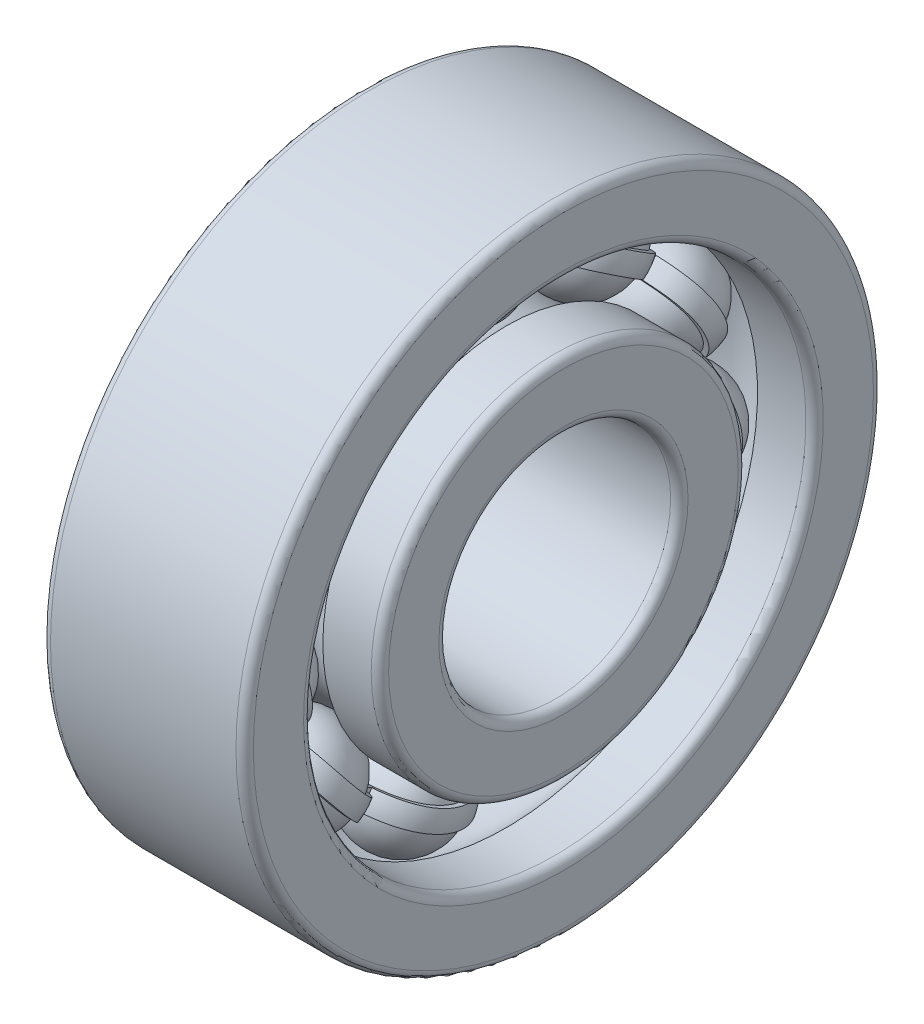
from build123d import *
from build123d.topology import SkipClean

# Parameters (mm, degrees)
SKETCH_5_W               = 1.05
SKETCH_5_H               = 0.7
PATTERN_CIRCULAR_5_COUNT = 11
PATTERN_CIRCULAR_2_COUNT = 11


with BuildPart() as part:
    # 草图2 → 旋转1 (revolve)
    with BuildSketch(Plane.XY, mode=Mode.PRIVATE) as revolve_1_sk:
        with BuildLine():
            Line((3.2, 4), (-3.2, 4))
            ThreePointArc((-3.2, 4), (-3.412132034, 4.087867966), (-3.5, 4.3))
            Line((-3.5, 4.3), (-3.5, 6.033333333))
            ThreePointArc((-3.5, 6.033333333), (-3.412132034, 6.245465368), (-3.2, 6.333333333))
            Line((-3.2, 6.333333333), (-1.304372987, 6.333333333))
            ThreePointArc((-1.304372987, 6.333333333), (0, 5.75), (1.304372987, 6.333333333))
            Line((1.304372987, 6.333333333), (3.2, 6.333333333))
            ThreePointArc((3.2, 6.333333333), (3.412132034, 6.245465368), (3.5, 6.033333333))
            Line((3.5, 6.033333333), (3.5, 4.3))
            ThreePointArc((3.5, 4.3), (3.412132034, 4.087867966), (3.2, 4))
        make_face()
        with BuildLine():
            Line((-3.5, 10.7), (-3.5, 8.966666667))
            ThreePointArc((-3.5, 8.966666667), (-3.412132034, 8.754534632), (-3.2, 8.666666667))
            Line((-3.2, 8.666666667), (-1.304372987, 8.666666667))
            ThreePointArc((-1.304372987, 8.666666667), (0, 9.25), (1.304372987, 8.666666667))
            Line((1.304372987, 8.666666667), (3.2, 8.666666667))
            ThreePointArc((3.2, 8.666666667), (3.412132034, 8.754534632), (3.5, 8.966666667))
            Line((3.5, 8.966666667), (3.5, 10.7))
            ThreePointArc((3.5, 10.7), (3.412132034, 10.912132034), (3.2, 11))
            Line((3.2, 11), (-3.2, 11))
            ThreePointArc((-3.2, 11), (-3.412132034, 10.912132034), (-3.5, 10.7))
        make_face()
    revolve(revolve_1_sk.sketch.rotate(Axis((-3.5, 0, 0), (1, 0, 0)), 90), axis=Axis((-3.5, 0, 0), (1, 0, 0)))


with BuildPart() as body_2:
    # 草图5 → 旋转3 (revolve)
    with BuildSketch(Plane.XY, mode=Mode.PRIVATE) as revolve_3_sk:
        with Locations((0, 7.5)):
            Rectangle(SKETCH_5_W, SKETCH_5_H)
    revolve(revolve_3_sk.sketch.rotate(Axis((-19.927092192, 0, 0), (1, 0, 0)), 90), axis=Axis((-19.927092192, 0, 0), (1, 0, 0)))



with BuildPart() as body_3:
    # 草图3 → 旋转2 (revolve)
    with BuildSketch(Plane.XY):
        with BuildLine():
            Line((-1.925, 7.5), (1.925, 7.5))
            ThreePointArc((1.925, 7.5), (0, 9.425), (-1.925, 7.5))
        make_face()
    revolve(axis=Axis((-1.925, 7.5, 0), (1, 0, 0)))


with BuildPart() as pattern_circular_5_1:
    # 阵列(圆周)5: pattern copy
    add(body_3.part.rotate(Axis((0, 0, 0), (1, 0, 0)), 1 * 360 / PATTERN_CIRCULAR_5_COUNT))


with BuildPart() as pattern_circular_5_2:
    # 阵列(圆周)5: pattern copy
    add(body_3.part.rotate(Axis((0, 0, 0), (1, 0, 0)), 2 * 360 / PATTERN_CIRCULAR_5_COUNT))


with BuildPart() as pattern_circular_5_3:
    # 阵列(圆周)5: pattern copy
    add(body_3.part.rotate(Axis((0, 0, 0), (1, 0, 0)), 3 * 360 / PATTERN_CIRCULAR_5_COUNT))


with BuildPart() as pattern_circular_5_4:
    # 阵列(圆周)5: pattern copy
    add(body_3.part.rotate(Axis((0, 0, 0), (1, 0, 0)), 4 * 360 / PATTERN_CIRCULAR_5_COUNT))


with BuildPart() as pattern_circular_5_5:
    # 阵列(圆周)5: pattern copy
    add(body_3.part.rotate(Axis((0, 0, 0), (1, 0, 0)), 5 * 360 / PATTERN_CIRCULAR_5_COUNT))


with BuildPart() as pattern_circular_5_6:
    # 阵列(圆周)5: pattern copy
    add(body_3.part.rotate(Axis((0, 0, 0), (1, 0, 0)), 6 * 360 / PATTERN_CIRCULAR_5_COUNT))


with BuildPart() as pattern_circular_5_7:
    # 阵列(圆周)5: pattern copy
    add(body_3.part.rotate(Axis((0, 0, 0), (1, 0, 0)), 7 * 360 / PATTERN_CIRCULAR_5_COUNT))


with BuildPart() as pattern_circular_5_8:
    # 阵列(圆周)5: pattern copy
    add(body_3.part.rotate(Axis((0, 0, 0), (1, 0, 0)), 8 * 360 / PATTERN_CIRCULAR_5_COUNT))


with BuildPart() as pattern_circular_5_9:
    # 阵列(圆周)5: pattern copy
    add(body_3.part.rotate(Axis((0, 0, 0), (1, 0, 0)), 9 * 360 / PATTERN_CIRCULAR_5_COUNT))


with BuildPart() as pattern_circular_5_10:
    # 阵列(圆周)5: pattern copy
    add(body_3.part.rotate(Axis((0, 0, 0), (1, 0, 0)), 10 * 360 / PATTERN_CIRCULAR_5_COUNT))


with BuildPart() as cut_revolve_1_tool:
    # 草图6 → 切除-旋转1 (revolve)
    with BuildSketch(Plane.XY):
        with BuildLine():
            Line((-1.89291442, 7.85), (1.89291442, 7.85))
            ThreePointArc((1.89291442, 7.85), (0, 9.425), (-1.89291442, 7.85))
        make_face()
        with BuildLine():
            Line((-1.89291442, 7.15), (1.89291442, 7.15))
            ThreePointArc((1.89291442, 7.15), (0, 5.575), (-1.89291442, 7.15))
        make_face()
    revolve(axis=Axis((-19.927092192, 0, 0), (1, 0, 0)))


with BuildPart() as part_1:
    add(part.part)

    # 切除-旋转1: cut by cut_revolve_1_tool
    add(cut_revolve_1_tool.part, mode=Mode.SUBTRACT)


with BuildPart() as body_3_1:
    add(body_3.part)

    # 切除-旋转1: cut by cut_revolve_1_tool
    add(cut_revolve_1_tool.part, mode=Mode.SUBTRACT)


with BuildPart() as pattern_circular_5_1_1:
    add(pattern_circular_5_1.part)

    # 切除-旋转1: cut by cut_revolve_1_tool
    add(cut_revolve_1_tool.part, mode=Mode.SUBTRACT)


with BuildPart() as pattern_circular_5_2_1:
    add(pattern_circular_5_2.part)

    # 切除-旋转1: cut by cut_revolve_1_tool
    add(cut_revolve_1_tool.part, mode=Mode.SUBTRACT)


with BuildPart() as pattern_circular_5_3_1:
    add(pattern_circular_5_3.part)

    # 切除-旋转1: cut by cut_revolve_1_tool
    add(cut_revolve_1_tool.part, mode=Mode.SUBTRACT)


with BuildPart() as pattern_circular_5_4_1:
    add(pattern_circular_5_4.part)

    # 切除-旋转1: cut by cut_revolve_1_tool
    add(cut_revolve_1_tool.part, mode=Mode.SUBTRACT)


with BuildPart() as pattern_circular_5_5_1:
    add(pattern_circular_5_5.part)

    # 切除-旋转1: cut by cut_revolve_1_tool
    add(cut_revolve_1_tool.part, mode=Mode.SUBTRACT)


with BuildPart() as pattern_circular_5_6_1:
    add(pattern_circular_5_6.part)

    # 切除-旋转1: cut by cut_revolve_1_tool
    add(cut_revolve_1_tool.part, mode=Mode.SUBTRACT)


with BuildPart() as pattern_circular_5_7_1:
    add(pattern_circular_5_7.part)

    # 切除-旋转1: cut by cut_revolve_1_tool
    add(cut_revolve_1_tool.part, mode=Mode.SUBTRACT)


with BuildPart() as pattern_circular_5_8_1:
    add(pattern_circular_5_8.part)

    # 切除-旋转1: cut by cut_revolve_1_tool
    add(cut_revolve_1_tool.part, mode=Mode.SUBTRACT)


with BuildPart() as pattern_circular_5_9_1:
    add(pattern_circular_5_9.part)

    # 切除-旋转1: cut by cut_revolve_1_tool
    add(cut_revolve_1_tool.part, mode=Mode.SUBTRACT)


with BuildPart() as pattern_circular_5_10_1:
    add(pattern_circular_5_10.part)

    # 切除-旋转1: cut by cut_revolve_1_tool
    add(cut_revolve_1_tool.part, mode=Mode.SUBTRACT)


with BuildPart() as body_2_1:
    with SkipClean():  # the faces are left unmerged after this step: merging them gives an invalid solid
        add(body_2.part)

        add(body_3_1.part)  # 旋转4 merges body 3
        # 草图7 → 旋转4 (revolve)
        with BuildSketch(Plane.XY):
            with BuildLine():
                Line((-1.75, 7.5), (1.75, 7.5))
                ThreePointArc((1.75, 7.5), (0, 9.25), (-1.75, 7.5))
            make_face()
        revolve_4 = revolve(axis=Axis((-1.75, 7.5, 0), (1, 0, 0)))

    # 阵列(圆周)2: 旋转4 ×11 about axis
    pattern_circular_2_axis = Axis((0, 0, 0), (1, 0, 0))
    for i in range(1, PATTERN_CIRCULAR_2_COUNT):
        add(revolve_4.rotate(pattern_circular_2_axis, i * 360 / PATTERN_CIRCULAR_2_COUNT))


solid = Compound([part_1.part, pattern_circular_5_1_1.part, pattern_circular_5_2_1.part, pattern_circular_5_3_1.part, pattern_circular_5_4_1.part, pattern_circular_5_5_1.part, pattern_circular_5_6_1.part, pattern_circular_5_7_1.part, pattern_circular_5_8_1.part, pattern_circular_5_9_1.part, pattern_circular_5_10_1.part, body_2_1.part])
